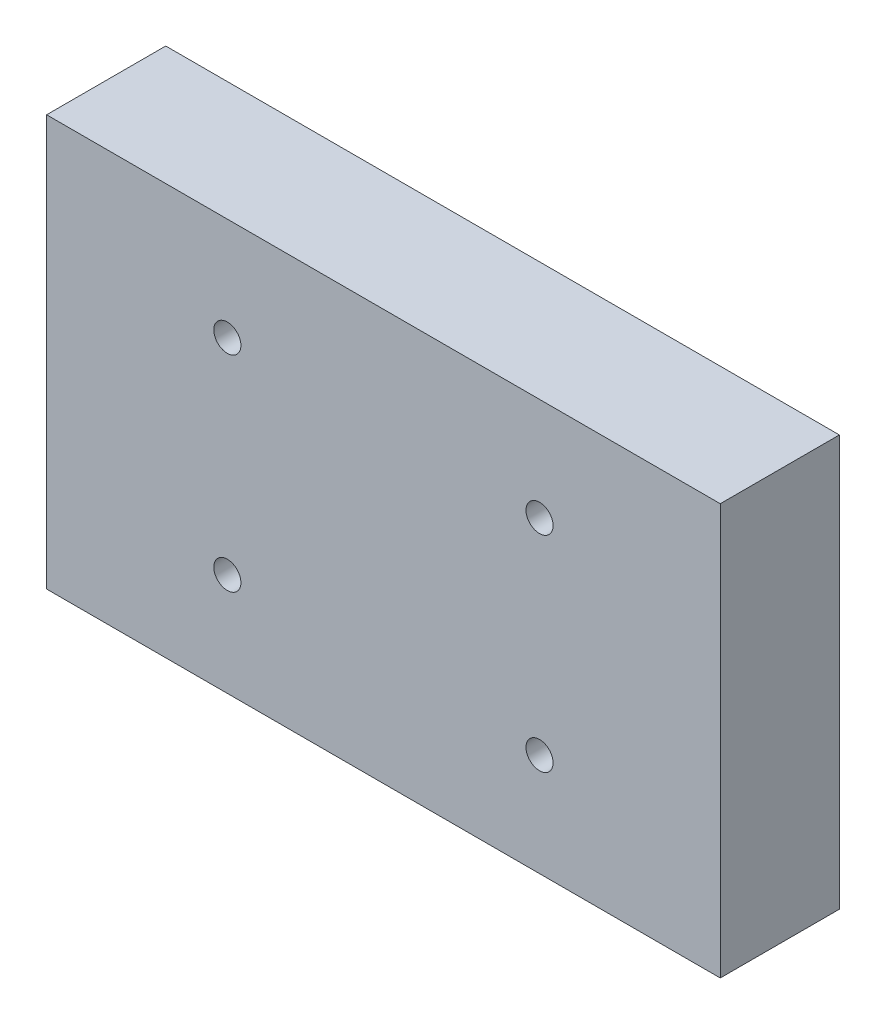
from build123d import *

# Parameters (mm, degrees)
SKETCH1_W            = 82
SKETCH1_H            = 50
BOSS_EXTRUDE1_DEPTH  = 16
M4_TAPPED_HOLE1_D    = 3.3
LPATTERN1_COUNT      = 2
LPATTERN1_PITCH      = 38
LPATTERN1_COUNT_DIR2 = 2
LPATTERN1_PITCH_DIR2 = 25
CHAMFER1_SIZE        = 1.5


with BuildPart() as part:
    # Sketch1 → Boss-Extrude1 (new body)
    with BuildSketch(Plane.XY):
        Rectangle(SKETCH1_W, SKETCH1_H)
    extrude(amount=BOSS_EXTRUDE1_DEPTH)

    # M4 Tapped Hole1 (through all)
    with Locations(Plane(origin=(19, 12.5, 0), x_dir=(-1, 0, 0), z_dir=(0, 0, -1))):
        with Locations((0, 0)):
            m4_tapped_hole1 = Hole(M4_TAPPED_HOLE1_D / 2)

    # LPattern1: M4 Tapped Hole1 2 × 2
    with Locations(*[(-i * LPATTERN1_PITCH, -j * LPATTERN1_PITCH_DIR2, 0) for i in range(LPATTERN1_COUNT) for j in range(LPATTERN1_COUNT_DIR2) if (i, j) != (0, 0)]):
        add(m4_tapped_hole1, mode=Mode.SUBTRACT)

    # Chamfer1
    chamfer1_edges = [part.edges().sort_by_distance(p)[0] for p in [
        (0, 25, 0),
        (41, 0, 0),
        (0, -25, 0),
        (-41, 0, 0),
    ]]
    chamfer(chamfer1_edges, length=CHAMFER1_SIZE)


solid = part.part
